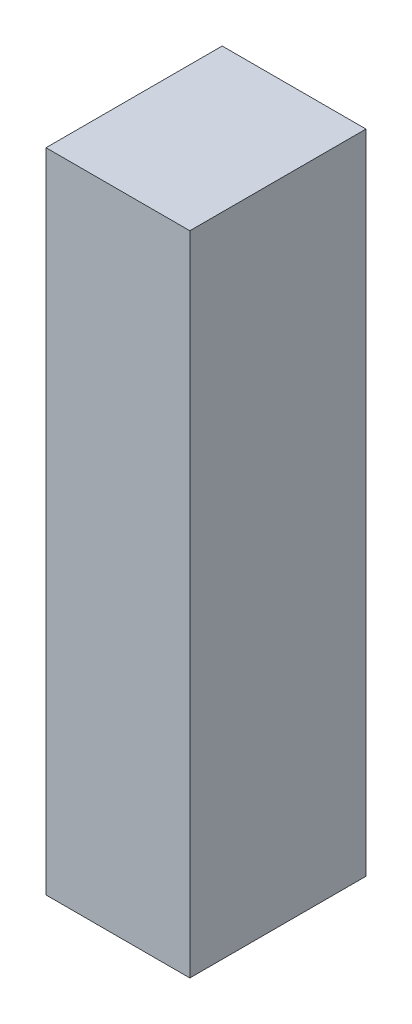
from build123d import *

# Parameters (mm, degrees)
SKETCH_1_W      = 20
SKETCH_1_H      = 90
EXTRUDE_1_DEPTH = 24.5


with BuildPart() as part:
    # 草图1 → 凸台-拉伸1 (new body)
    with BuildSketch(Plane.XY):
        with Locations((10, 0)):
            Rectangle(SKETCH_1_W, SKETCH_1_H)
    extrude(amount=EXTRUDE_1_DEPTH)


solid = part.part
